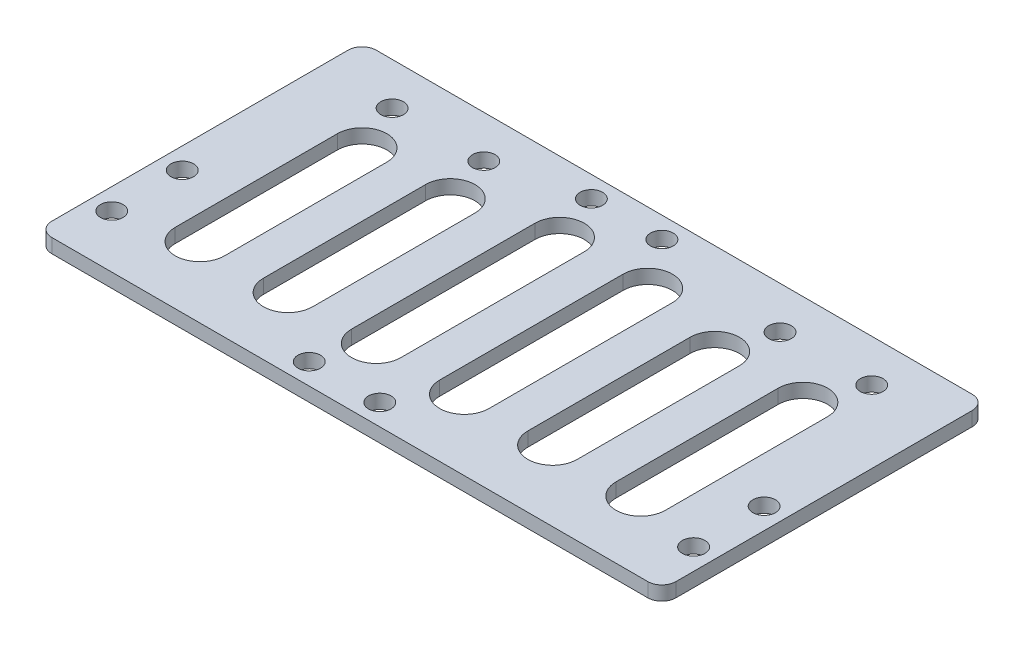
from build123d import *

# Parameters (mm, degrees)
SKETCH1_W           = 88.5
SKETCH1_H           = 46
SKETCH1_R           = 1.6
BOSS_EXTRUDE1_DEPTH = 2
CUT_EXTRUDE1_DEPTH  = 50.910544978
FILLET1_R           = 2


with BuildPart() as part:
    # Sketch1 → Boss-Extrude1 (new body)
    with BuildSketch(Plane(origin=(0, 0, 0), x_dir=(1, 0, 0), z_dir=(0, 1, 0))):
        Rectangle(SKETCH1_W, SKETCH1_H)
        with Locations(Location((-41.25, -5.5, 0), (0, 0, 270))):
            Circle(SKETCH1_R, mode=Mode.SUBTRACT)
        with Locations(Location((-41.25, -15.5, 0), (0, 0, 270))):
            Circle(SKETCH1_R, mode=Mode.SUBTRACT)
        with Locations(Location((41.25, -15.5, 0), (0, 0, 90))):
            Circle(SKETCH1_R, mode=Mode.SUBTRACT)
        with Locations(Location((41.25, -5.5, 0), (0, 0, 90))):
            Circle(SKETCH1_R, mode=Mode.SUBTRACT)
        with Locations(Location((-8.75, -20, 0), (0, 0, 270))):
            Circle(SKETCH1_R, mode=Mode.SUBTRACT)
        with Locations(Location((1.25, -20, 0), (0, 0, 270))):
            Circle(SKETCH1_R, mode=Mode.SUBTRACT)
        with Locations(Location((-34, 17, 0), (0, 0, 270))):
            Circle(SKETCH1_R, mode=Mode.SUBTRACT)
        with Locations(Location((-21, 17, 0), (0, 0, 270))):
            Circle(SKETCH1_R, mode=Mode.SUBTRACT)
        with Locations(Location((21, 17, 0), (0, 0, 270))):
            Circle(SKETCH1_R, mode=Mode.SUBTRACT)
        with Locations(Location((34, 17, 0), (0, 0, 270))):
            Circle(SKETCH1_R, mode=Mode.SUBTRACT)
        with Locations(Location((1.25, 20, 0), (0, 0, 90))):
            Circle(SKETCH1_R, mode=Mode.SUBTRACT)
        with Locations(Location((-8.75, 20, 0), (0, 0, 90))):
            Circle(SKETCH1_R, mode=Mode.SUBTRACT)
    extrude(amount=BOSS_EXTRUDE1_DEPTH)

    # Sketch2 → Cut-Extrude1 (cut, through all)
    with BuildSketch(Plane(origin=(0, 2, 0), x_dir=(1, 0, 0), z_dir=(0, 1, 0))):
        with BuildLine():
            Line((-27.75, 10), (-27.75, -13))
            ThreePointArc((-27.75, -13), (-31.25, -16.5), (-34.75, -13))
            Line((-34.75, -13), (-34.75, 10))
            ThreePointArc((-34.75, 10), (-31.25, 13.5), (-27.75, 10))
        make_face()
        with BuildLine():
            Line((-15.25, 10), (-15.25, -13))
            ThreePointArc((-15.25, -13), (-18.75, -16.5), (-22.25, -13))
            Line((-22.25, -13), (-22.25, 10))
            ThreePointArc((-22.25, 10), (-18.75, 13.5), (-15.25, 10))
        make_face()
        with BuildLine():
            Line((-2.75, 13), (-2.75, -13))
            ThreePointArc((-2.75, -13), (-6.25, -16.5), (-9.75, -13))
            Line((-9.75, -13), (-9.75, 13))
            ThreePointArc((-9.75, 13), (-6.25, 16.5), (-2.75, 13))
        make_face()
        with BuildLine():
            Line((9.75, 13), (9.75, -13))
            ThreePointArc((9.75, -13), (6.25, -16.5), (2.75, -13))
            Line((2.75, -13), (2.75, 13))
            ThreePointArc((2.75, 13), (6.25, 16.5), (9.75, 13))
        make_face()
        with BuildLine():
            Line((22.25, 10), (22.25, -13))
            ThreePointArc((22.25, -13), (18.75, -16.5), (15.25, -13))
            Line((15.25, -13), (15.25, 10))
            ThreePointArc((15.25, 10), (18.75, 13.5), (22.25, 10))
        make_face()
        with BuildLine():
            Line((34.75, 10), (34.75, -13))
            ThreePointArc((34.75, -13), (31.25, -16.5), (27.75, -13))
            Line((27.75, -13), (27.75, 10))
            ThreePointArc((27.75, 10), (31.25, 13.5), (34.75, 10))
        make_face()
    extrude(amount=-CUT_EXTRUDE1_DEPTH, mode=Mode.SUBTRACT)

    # Fillet1
    fillet1_edges = [part.edges().sort_by_distance(p)[0] for p in [
        (44.25, 1, 23),
        (-44.25, 1, 23),
        (-44.25, 1, -23),
        (44.25, 1, -23),
    ]]
    fillet(fillet1_edges, radius=FILLET1_R)


solid = part.part
